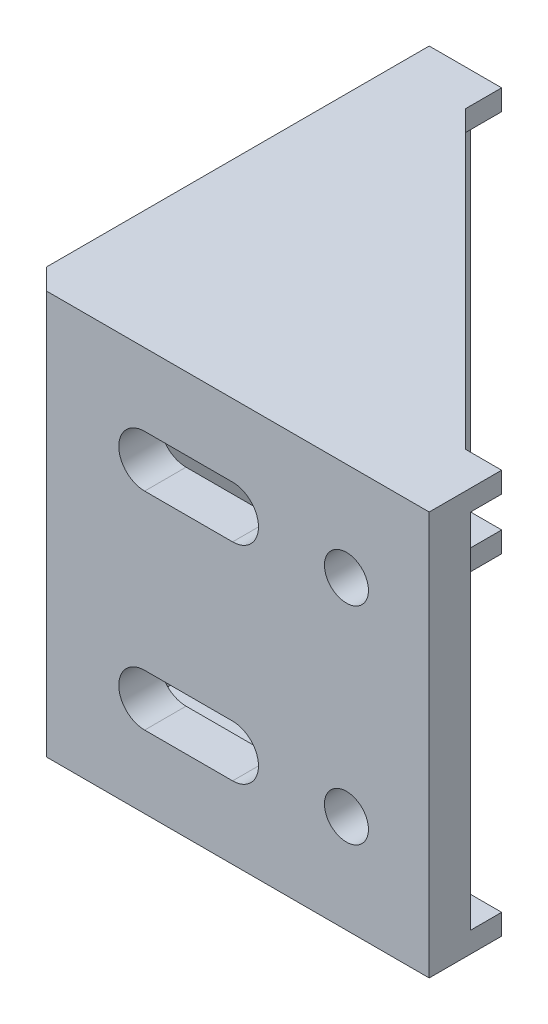
from build123d import *

# Parameters (mm, degrees)
BOSS_EXTRUDE1_DEPTH            = 74
SKETCH2_W                      = 64
SKETCH2_H                      = 74
BOSS_EXTRUDE2_DEPTH            = 14
SKETCH3_W                      = 64
SKETCH3_H                      = 78
BOSS_EXTRUDE3_DEPTH            = 4
CUT_EXTRUDE1_DEPTH             = 70
SKETCH5_W                      = 78
SKETCH5_H                      = 78
BOSS_EXTRUDE4_DEPTH            = 14
CUT_EXTRUDE2_REACH             = 115.771
SKETCH7_W                      = 64
SKETCH7_H                      = 70
CUT_EXTRUDE3_REACH             = 124.581
SKETCH9_W                      = 70
SKETCH9_H                      = 70
CUT_EXTRUDE4_DEPTH             = 110.936081615
CUT_EXTRUDE5_DEPTH             = 123.581337469
CUT_EXTRUDE6_DEPTH             = 119.860244595
CUT_EXTRUDE7_DEPTH             = 119.860244595
CUT_EXTRUDE8_DEPTH             = 128.31922202
F_8_5_8_5_DIAMETER_HOLE1_D     = 8.5
F_8_5_8_5_DIAMETER_HOLE1_DEPTH = 78
F_8_5_8_5_DIAMETER_HOLE2_D     = 8.5
F_8_5_8_5_DIAMETER_HOLE2_DEPTH = 78
CHAMFER1_SIZE                  = 4


with BuildPart() as part:
    # Sketch1 → Boss-Extrude1 (new body)
    with BuildSketch(Plane(origin=(0, 78, 0), x_dir=(1, 0, 0), z_dir=(0, 1, 0))):
        Polygon((-19.730848831, -49.578174681), (37.269151169, -49.578174681), (-19.730848831, 7.421825319), align=None)
    extrude(amount=-BOSS_EXTRUDE1_DEPTH)

    # Sketch2 → Boss-Extrude2 (add)
    with BuildSketch(Plane.XY.offset(49.578174681)):
        with Locations((12.269151169, 41)):
            Rectangle(SKETCH2_W, SKETCH2_H)
    extrude(amount=BOSS_EXTRUDE2_DEPTH)

    # Sketch3 → Boss-Extrude3 (add)
    with BuildSketch(Plane.XZ.offset(-4)):
        with Locations((12.269151169, 24.578174681)):
            Rectangle(SKETCH3_W, SKETCH3_H)
    extrude(amount=BOSS_EXTRUDE3_DEPTH)

    # Sketch4 → Cut-Extrude1 (cut)
    with BuildSketch(Plane.XZ.offset(-4)):
        Polygon((-19.730848831, -7.421825319), (37.269151169, 49.578174681), (-19.730848831, 49.578174681), align=None)
    extrude(amount=-CUT_EXTRUDE1_DEPTH, mode=Mode.SUBTRACT)

    # Sketch5 → Boss-Extrude4 (add)
    with BuildSketch(Plane.ZY.offset(19.730848831)):
        with Locations((24.578174681, 39)):
            Rectangle(SKETCH5_W, SKETCH5_H)
    extrude(amount=BOSS_EXTRUDE4_DEPTH)

    # Sketch7 → Cut-Extrude2 (cut, up to next)
    with BuildSketch(Plane.XY.offset(55.578174681), mode=Mode.PRIVATE) as cut_extrude2_sk1:
        with Locations((12.269151169, 39)):
            Rectangle(SKETCH7_W, SKETCH7_H)
    cut_extrude2_tool1 = extrude(cut_extrude2_sk1.sketch, amount=-CUT_EXTRUDE2_REACH, mode=Mode.PRIVATE) & part.part
    add(cut_extrude2_tool1.solids().sort_by_distance((12.269151, 39, 55.578175))[0], mode=Mode.SUBTRACT)

    # Sketch9 → Cut-Extrude3 (cut, up to next)
    with BuildSketch(Plane(origin=(-25.730848831, 0, 0), x_dir=(0, -1, 0), z_dir=(-1, 0, 0)), mode=Mode.PRIVATE) as cut_extrude3_sk1:
        with Locations((-39, 20.578174681)):
            Rectangle(SKETCH9_W, SKETCH9_H)
    cut_extrude3_tool1 = extrude(cut_extrude3_sk1.sketch, amount=-CUT_EXTRUDE3_REACH, mode=Mode.PRIVATE) & part.part
    add(cut_extrude3_tool1.solids().sort_by_distance((-25.730849, 39, 20.578175))[0], mode=Mode.SUBTRACT)

    # Sketch10 → Cut-Extrude4 (cut, through all)
    with BuildSketch(Plane.XZ):
        Polygon((44.269151169, 49.578174681), (37.269151169, 49.578174681), (-19.730848831, -7.421825319), (-19.730848831, -14.421825319), (44.269151169, -14.421825319), align=None)
    extrude(amount=-CUT_EXTRUDE4_DEPTH, mode=Mode.SUBTRACT)

    # Sketch11 → Cut-Extrude5 (cut, through all)
    with BuildSketch(Plane(origin=(-25.730848831, 0, 0), x_dir=(0, 0, -1), z_dir=(1, 0, 0))):
        with BuildLine():
            Line((-23.578174681, 24), (-40.578174681, 24))
            ThreePointArc((-40.578174681, 24), (-45.578174681, 19), (-40.578174681, 14))
            Line((-40.578174681, 14), (-23.578174681, 14))
            ThreePointArc((-23.578174681, 14), (-18.578174681, 19), (-23.578174681, 24))
        make_face()
    extrude(amount=-CUT_EXTRUDE5_DEPTH, mode=Mode.SUBTRACT)

    # Sketch12 → Cut-Extrude6 (cut, through all)
    with BuildSketch(Plane.XY.offset(63.578174681)):
        with BuildLine():
            Line((6.269151169, 64), (-10.730848831, 64))
            ThreePointArc((-10.730848831, 64), (-15.730848831, 59), (-10.730848831, 54))
            Line((-10.730848831, 54), (6.269151169, 54))
            ThreePointArc((6.269151169, 54), (11.269151169, 59), (6.269151169, 64))
        make_face()
    extrude(amount=-CUT_EXTRUDE6_DEPTH, mode=Mode.SUBTRACT)

    # Sketch13 → Cut-Extrude7 (cut, through all)
    with BuildSketch(Plane.XY.offset(63.578174681)):
        with BuildLine():
            Line((6.269151169, 24), (-10.730848831, 24))
            ThreePointArc((-10.730848831, 24), (-15.730848831, 19), (-10.730848831, 14))
            Line((-10.730848831, 14), (6.269151169, 14))
            ThreePointArc((6.269151169, 14), (11.269151169, 19), (6.269151169, 24))
        make_face()
    extrude(amount=-CUT_EXTRUDE7_DEPTH, mode=Mode.SUBTRACT)

    # Sketch14 → Cut-Extrude8 (cut, through all)
    with BuildSketch(Plane.ZY.offset(33.730848831)):
        with BuildLine():
            Line((23.078174681, 54), (40.078174681, 54))
            ThreePointArc((40.078174681, 54), (45.078174681, 59), (40.078174681, 64))
            Line((40.078174681, 64), (23.078174681, 64))
            ThreePointArc((23.078174681, 64), (18.078174681, 59), (23.078174681, 54))
        make_face()
    extrude(amount=-CUT_EXTRUDE8_DEPTH, mode=Mode.SUBTRACT)

    # Ø8.5 (8.5) Diameter Hole1
    with Locations(Plane.ZY.offset(33.730848831)):
        with Locations((1.578174681, 59), (1.578174681, 19)):
            Hole(F_8_5_8_5_DIAMETER_HOLE1_D / 2, depth=F_8_5_8_5_DIAMETER_HOLE1_DEPTH)

    # Ø8.5 (8.5) Diameter Hole2
    with Locations(Plane.XY.offset(63.578174681)):
        with Locations((28.269151169, 19), (28.269151169, 59)):
            Hole(F_8_5_8_5_DIAMETER_HOLE2_D / 2, depth=F_8_5_8_5_DIAMETER_HOLE2_DEPTH)

    # Chamfer1
    chamfer1_edges = [part.edges().sort_by_distance(p)[0] for p in [
        (-33.730848831, 39, 63.578174681),
    ]]
    chamfer(chamfer1_edges, length=CHAMFER1_SIZE)


solid = part.part
